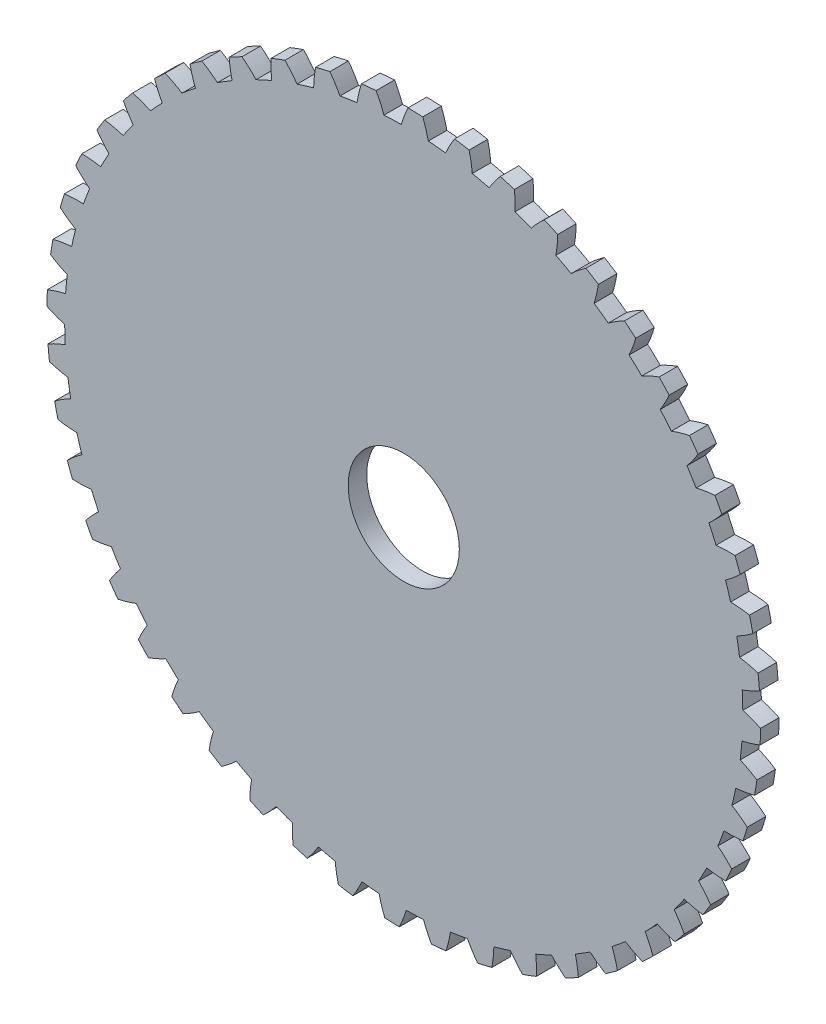
SolidWorks part; units mm, degrees
ref_plane "Front Plane" through (0, 0, 0) normal (0, 0, 1) x (1, 0, 0)
ref_plane "Top Plane" through (0, 0, 0) normal (0, 1, 0) x (1, 0, 0)
ref_plane "Right Plane" through (0, 0, 0) normal (1, 0, 0) x (0, 0, -1)
sketch "Sketch1" plane through (0, 0, 0) normal (0, 0, 1) x (1, 0, 0)
  circle A0 centre (0, 0) radius 9.15
  dimension "D1" = 18.3
extrude "Boss-Extrude1" add sketch "Sketch1" along normal blind 0.5
sketch "Sketch2" plane through (0, 0, 0.5) normal (0, 0, 1) x (1, 0, 0)
  line L0 (0, 0) -> (0, 11.5553) construction
  line L1 (0, 0) -> (0.386, 11.792) construction
  line L2 (0, 0) -> (4.1863, 11.5017) construction
  line L3 (0, 9.35) -> (3.005, 8.2563) construction
  circle A0 centre (0, 0) radius 9.35 construction
  circle A1 centre (0, 0) radius 9.63 construction
  arc A2 (0.1169, 9.6293) -> (-0.0655, 9.1498) centre (3.005, 8.2563) ccw
  arc A3 (0.6638, 9.1259) -> (-0.0655, 9.1498) centre (0, 0) ccw
  arc A4 (9.2092, 2.8155) -> (3.2937, 9.0492) centre (0, 0) ccw
  arc A5 (0.5131, 9.6163) -> (0.6638, 9.1259) centre (-2.4586, 8.4351) cw
  arc A6 (0.5131, 9.6163) -> (0, 9.63) centre (0, 0) ccw
  circle M8 centre (0, 0) radius 9.15
  dimension "D1" = 18.7
  dimension "D2" = 19.26
  dimension "D3" = 20
  dimension "D4" = 1.875
extrude "Boss-Extrude2" add sketch "Sketch2" against normal blind 0.5 contours A5 A6 A2 M8
pattern_circular "CirPattern1" count 48 over 360 about axis through (0, 0, 0) along (0, 0, 1) of "Boss-Extrude2"
sketch "Sketch3" plane through (0, 0, 0.5) normal (0, 0, 1) x (1, 0, 0)
  circle A0 centre (0, 0) radius 1.5
  dimension "D1" = 3
extrude "Cut-Extrude1" cut sketch "Sketch3" against normal blind 5
